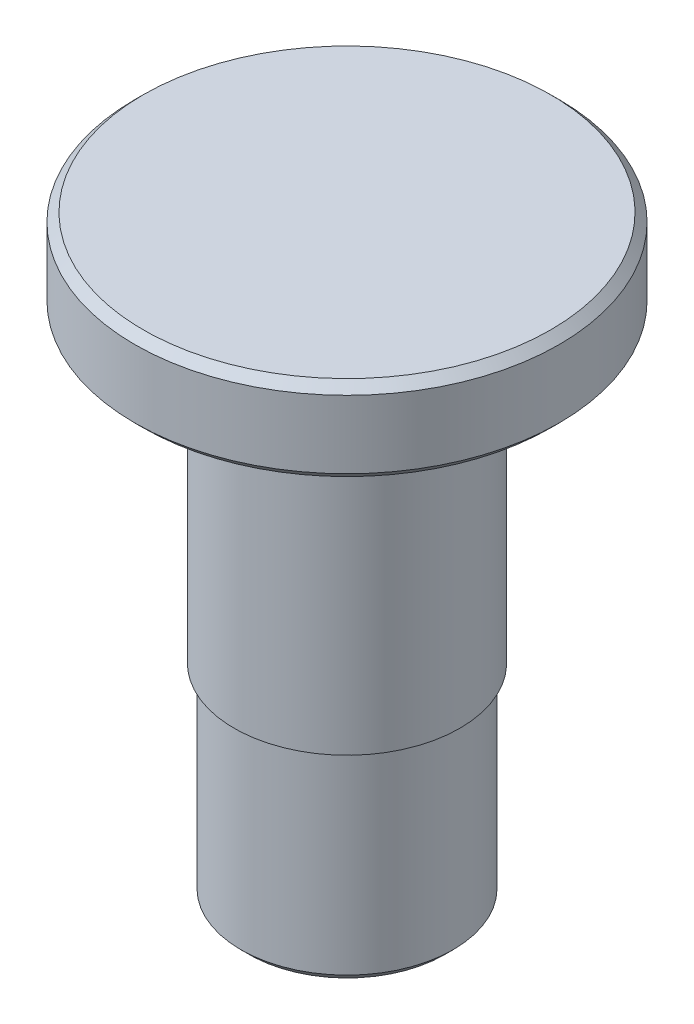
from build123d import *

# Parameters (mm, degrees)
CHAMFER1_SIZE = 0.5


with BuildPart() as part:
    # Sketch1 → Revolve1 (revolve)
    with BuildSketch(Plane.XY):
        Polygon((-139.286891893, -435.685707644), (-139.686891893, -435.685707644), (-139.686891893, -417.685707644), (-145.536891893, -417.685707644), (-145.536891893, -412.685707644), (-133.036891893, -412.685707644), (-133.036891893, -447.685707644), (-139.286891893, -447.685707644), align=None)
    revolve(axis=Axis((-133.036891893, -412.685707644, 0), (0, -1, 0)))

    # Chamfer1
    chamfer1_edges = [part.edges().sort_by_distance(p)[0] for p in [
        (-120.536891893, -412.685707644, 0),
        (-120.536891893, -417.685707644, 0),
        (-126.786891893, -447.685707644, 0),
    ]]
    chamfer(chamfer1_edges, length=CHAMFER1_SIZE)


solid = part.part
